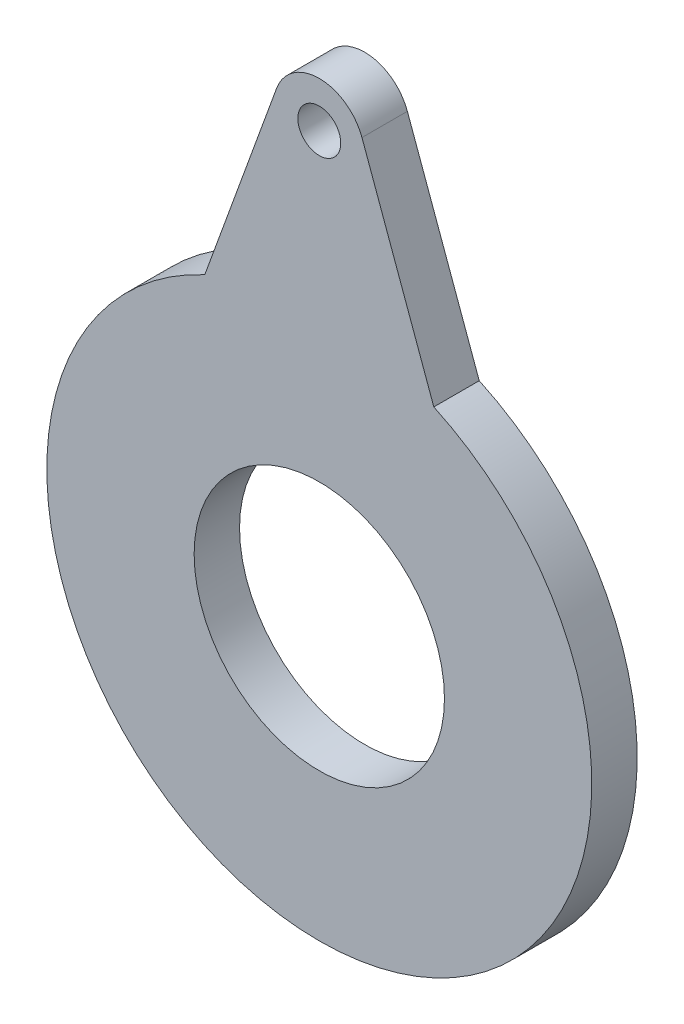
SolidWorks part; units mm, degrees
ref_plane "Front Plane" through (0, 0, 0) normal (0, 0, 1) x (1, 0, 0)
ref_plane "Top Plane" through (0, 0, 0) normal (0, 1, 0) x (1, 0, 0)
ref_plane "Right Plane" through (0, 0, 0) normal (1, 0, 0) x (0, 0, -1)
sketch "Sketch1" plane through (0, 0, 222.25) normal (0, 0, 1) x (1, 0, 0)
  line L0 (0, 0) -> (0, 90) construction
  line L1 (-8.9506, 93.2577) -> (-24.019, 51.8576)
  line L2 (8.9506, 93.2577) -> (24.019, 51.8576)
  circle A0 centre (0, 0) radius 57.15 construction
  arc A1 (-24.019, 51.8576) -> (24.019, 51.8576) centre (0, 0) ccw
  circle A2 centre (0, 0) radius 26.2509 construction
  circle A3 centre (0, 0) radius 26.2509
  circle A4 centre (0, 0) radius 90 construction
  arc A5 (8.9506, 93.2577) -> (-8.9506, 93.2577) centre (0, 90) ccw
  circle A6 centre (0, 90) radius 4.5
  dimension "D1" = 180
  dimension "D3" = 19.05
  dimension "D4" = 9
  dimension "D2" = 40
extrude "Boss-Extrude1" add sketch "Sketch1" along normal blind 9.525
